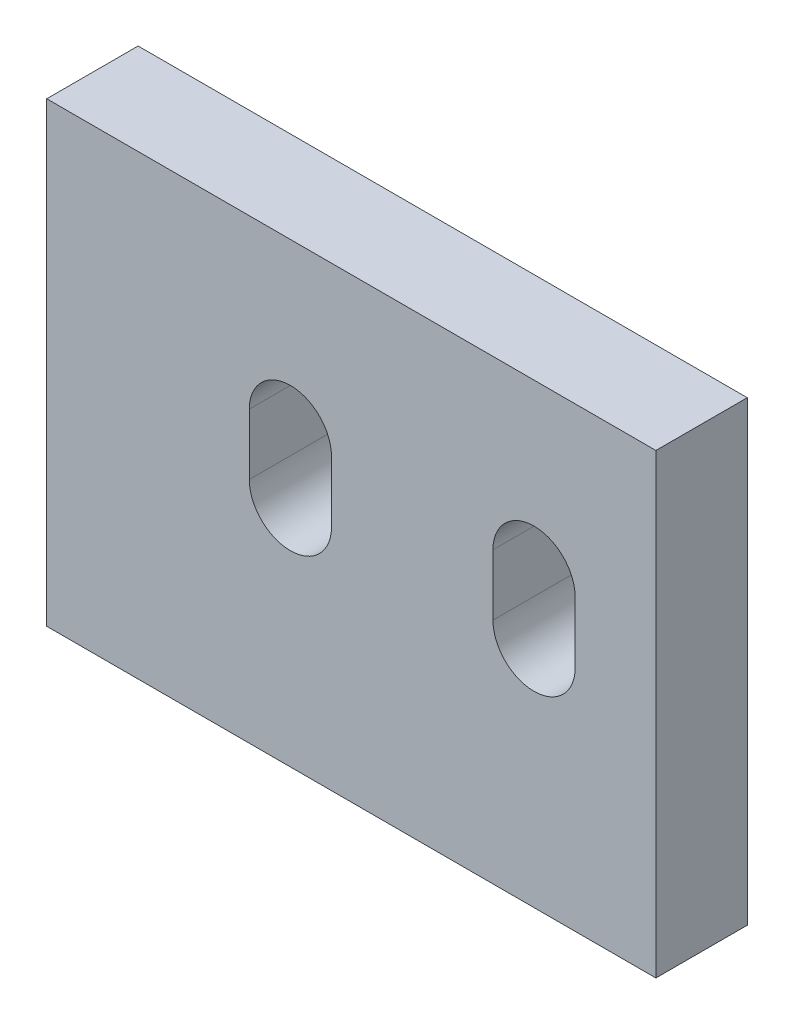
from build123d import *

# Parameters (mm, degrees)
SKETCH1_W           = 200
SKETCH1_H           = 150
BOSS_EXTRUDE1_DEPTH = 30


with BuildPart() as part:
    # Sketch1 → Boss-Extrude1 (new body)
    with BuildSketch(Plane.XY):
        with Locations((100, 75)):
            Rectangle(SKETCH1_W, SKETCH1_H)
        with BuildLine():
            Line((93.5, 95), (93.5, 75))
            ThreePointArc((93.5, 75), (80, 61.5), (66.5, 75))
            Line((66.5, 75), (66.5, 95))
            ThreePointArc((66.5, 95), (80, 108.5), (93.5, 95))
        make_face(mode=Mode.SUBTRACT)
        with BuildLine():
            Line((173.5, 95), (173.5, 75))
            ThreePointArc((173.5, 75), (160, 61.5), (146.5, 75))
            Line((146.5, 75), (146.5, 95))
            ThreePointArc((146.5, 95), (160, 108.5), (173.5, 95))
        make_face(mode=Mode.SUBTRACT)
    extrude(amount=BOSS_EXTRUDE1_DEPTH)


solid = part.part
